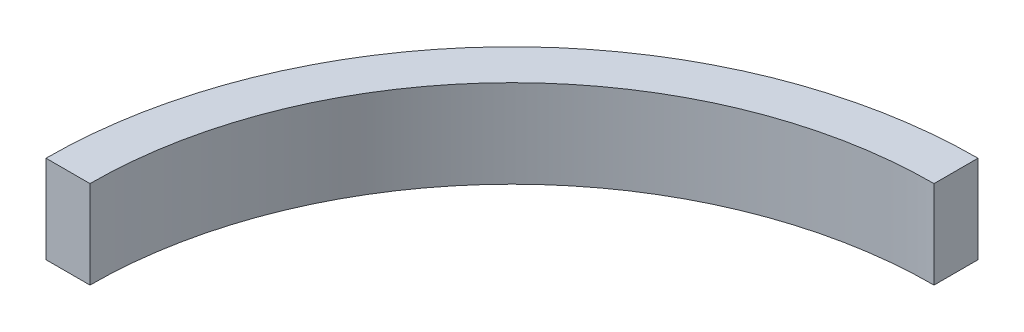
from build123d import *

# Parameters (mm, degrees)
EXTRUDE_1_DEPTH = 30


with BuildPart() as part:
    # 草图1 → 凸台-拉伸1 (new body)
    with BuildSketch(Plane(origin=(0, 0, 0), x_dir=(1, 0, 0), z_dir=(0, 1, 0))):
        with BuildLine():
            Line((-159, 0), (-144, 0))
            ThreePointArc((-144, 0), (-101.823376491, 101.823376491), (0, 144))
            Line((0, 144), (0, 159))
            ThreePointArc((0, 159), (-112.429978209, 112.429978209), (-159, 0))
        make_face()
    extrude(amount=EXTRUDE_1_DEPTH)


solid = part.part
